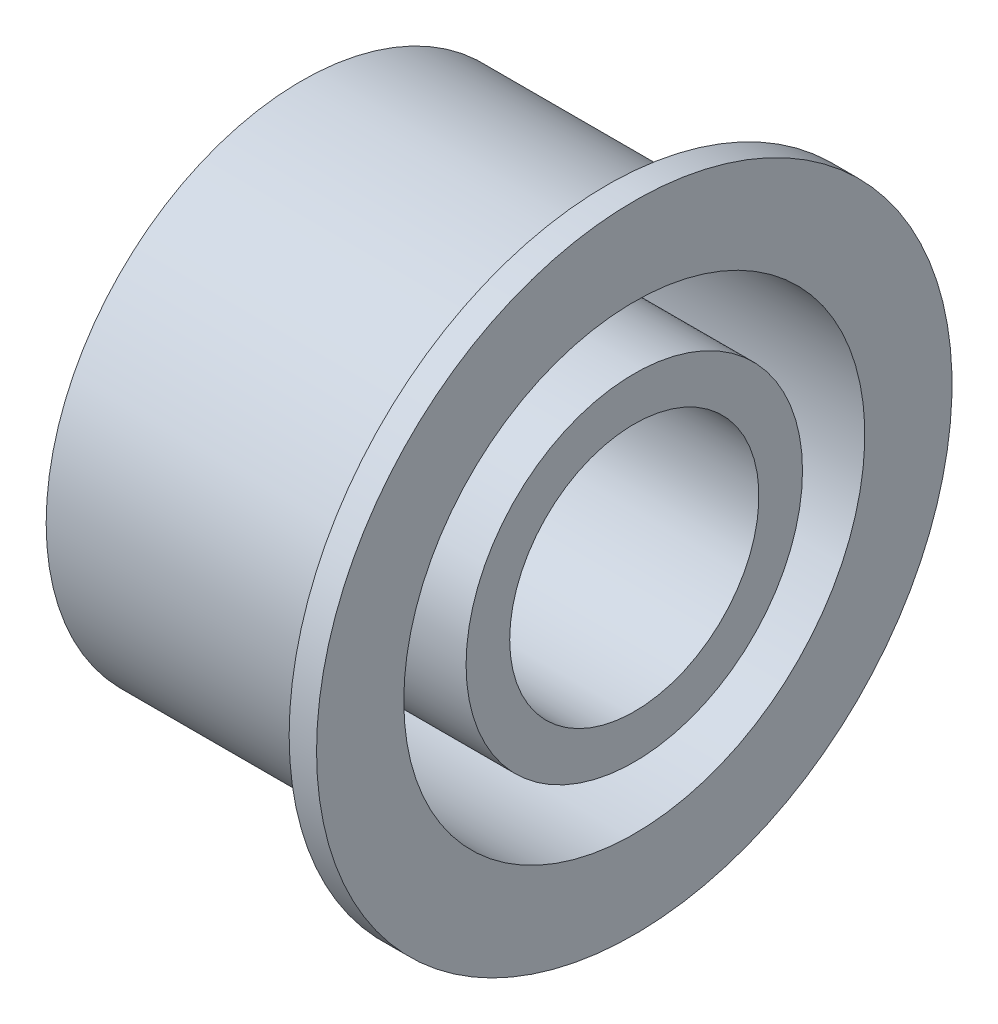
from build123d import *


with BuildPart() as part:
    # 草图1 → 旋转1 (revolve)
    with BuildSketch(Plane.XY, mode=Mode.PRIVATE) as revolve_1_sk:
        Polygon((25.3, 25.5), (25.3, 20.5), (0.8, 20.5), (0.8, 13.5), (0, 13.5), (0, 10), (27.5, 10), (27.5, 13.5), (4.3, 13.5), (4.3, 18.5), (27.5, 18.5), (27.5, 25.5), align=None)
    revolve(revolve_1_sk.sketch.rotate(Axis((0, 0, 0), (1, 0, 0)), 90), axis=Axis((0, 0, 0), (1, 0, 0)))


solid = part.part
